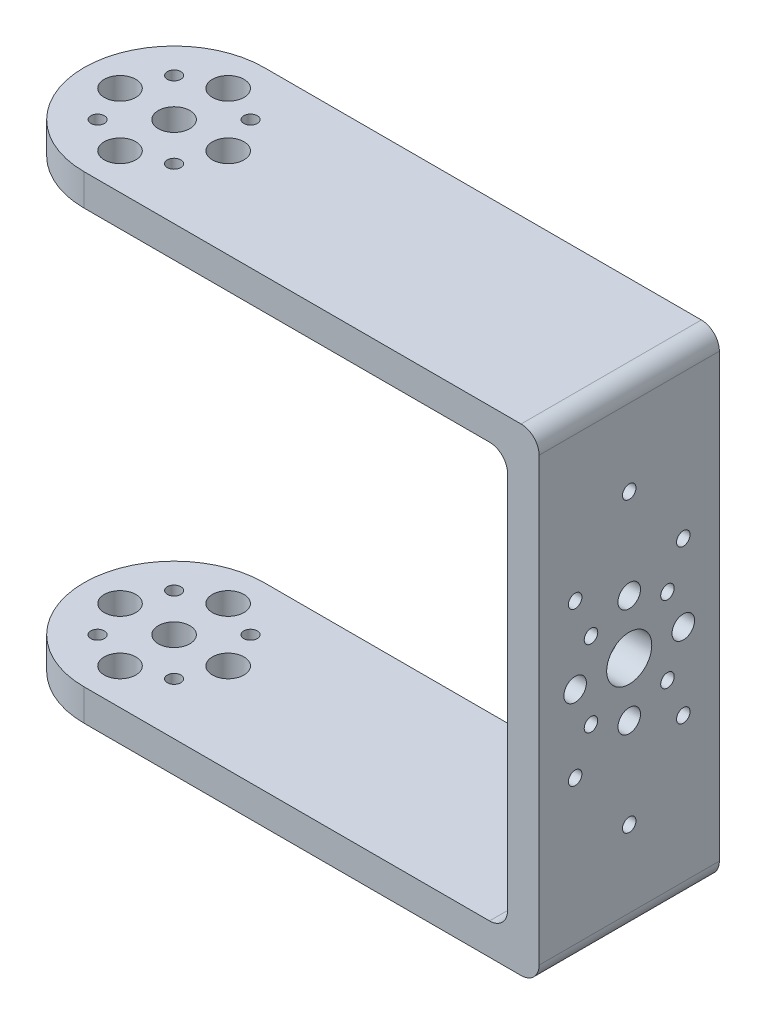
SolidWorks part; units mm, degrees
material "45"
ref_plane "Front Plane" through (0, 0, 0) normal (0, 0, 1) x (1, 0, 0)
ref_plane "Top Plane" through (0, 0, 0) normal (0, 1, 0) x (1, 0, 0)
ref_plane "Right Plane" through (0, 0, 0) normal (1, 0, 0) x (0, 0, -1)
sketch "Sketch2" plane through (0, 0, 0) normal (0, 0, 1) x (1, 0, 0)
  line L0 (4.8689, 24.8459) -> (4.8689, 28.3459)
  line L2 (4.8689, 28.3459) -> (65.3689, 28.3459)
  line L3 (4.8689, 24.8459) -> (61.8689, 24.8459)
  line L4 (4.8689, -21.1541) -> (4.8689, -24.6541)
  line L6 (4.8689, -21.1541) -> (61.8689, -21.1541)
  line L7 (4.8689, -24.6541) -> (65.3689, -24.6541)
  line L8 (65.3689, -24.6541) -> (65.3689, 28.3459)
  line L9 (61.8689, 24.8459) -> (61.8689, -21.1541)
  dimension "D1" = 3.5
  dimension "D2" = 3.5
  dimension "D3" = 3.5
  dimension "D4" = 57
extrude "Boss-Extrude1" add sketch "Sketch2" against normal blind 20
sketch "Sketch3" plane through (0, 28.3459, 0) normal (0, 1, 0) x (1, 0, 0)
  line L0 (4.8689, 10) -> (25.951, 10) construction
  line L1 (4.8689, 20) -> (4.8689, 0) construction
  line L2 (14.8689, 20) -> (4.8689, 20)
  line L3 (4.8689, 20) -> (4.8689, 10)
  line L4 (4.8689, 10) -> (4.8689, 0)
  line L5 (4.8689, 0) -> (14.8689, 0)
  arc A0 (14.8689, 20) -> (14.8689, 0) centre (14.8689, 10) ccw
  line M2 (4.8689, 0) -> (65.3689, 0)
  line M4 (65.3689, 20) -> (4.8689, 20)
  line M5 (4.8689, 20) -> (4.8689, 0)
extrude "Cut-Extrude1" cut sketch "Sketch3" against normal through all contours A0 M5 M2 | A0 M4 M5
sketch "Sketch5" plane through (0, 28.3459, 0) normal (0, 1, 0) x (1, 0, 0)
  circle A0 centre (14.8689, 10) radius 1.75
  circle A1 centre (14.8689, 10) radius 6 construction
  circle A2 centre (20.8689, 10) radius 1.75
  circle A3 centre (14.8689, 4) radius 1.75
  circle A4 centre (8.8689, 10) radius 1.75
  circle A5 centre (14.8689, 16) radius 1.75
  circle A6 centre (19.1115, 5.7574) radius 0.75
  circle A7 centre (10.6262, 5.7574) radius 0.75
  circle A8 centre (10.6262, 14.2426) radius 0.75
  circle A9 centre (19.1115, 14.2426) radius 0.75
  point P15 (14.8689, 10)
  point P24 (14.8689, 10)
  dimension "D1" = 3.5
  dimension "D2" = 12
  dimension "D3" = 3.5
  dimension "D5" = 1.5
  dimension "D4" = 4
  dimension "D6" = 4
extrude "Cut-Extrude2" cut sketch "Sketch5" against normal through all
fillet "Fillet1" radius 2 2 edges at (65.3689, -24.6541, -10) (65.3689, 28.3459, -10)
sketch "Sketch6" plane through (65.3689, 0, 0) normal (1, 0, 0) x (0, 0, -1)
  line L0 (0, 1.8459) -> (20, 1.8459) construction
  line L1 (0, -22.6541) -> (0, 26.3459) construction
  line L2 (20, -22.6541) -> (20, 26.3459) construction
  circle A0 centre (10, 1.8459) radius 6 construction
  circle A1 centre (10, 1.8459) radius 2.5
  circle A2 centre (10, 7.8459) radius 1.25
  circle A3 centre (16, 1.8459) radius 1.25
  circle A4 centre (10, -4.1541) radius 1.25
  circle A5 centre (4, 1.8459) radius 1.25
  circle A6 centre (14.2426, 6.0885) radius 0.75
  circle A7 centre (14.2426, -2.3968) radius 0.75
  circle A8 centre (5.7574, -2.3968) radius 0.75
  circle A9 centre (5.7574, 6.0885) radius 0.75
  point P20 (10, 1.8459)
  point P29 (10, 1.8459)
  dimension "D1" = 12
  dimension "D2" = 5
  dimension "D3" = 2.5
  dimension "D5" = 1.5
  dimension "D4" = 4
  dimension "D6" = 4
extrude "Cut-Extrude3" cut sketch "Sketch6" against normal blind 20
sketch "Sketch7" plane through (65.3689, 0, 0) normal (1, 0, 0) x (0, 0, -1)
  line L1 (16, -6.6541) -> (4, -6.6541) construction
  line L2 (16, -6.6541) -> (16, 10.3459) construction
  line L3 (16, 10.3459) -> (4, 10.3459) construction
  line L4 (4, -6.6541) -> (4, 10.3459) construction
  line L5 (16, -6.6541) -> (4, 10.3459) construction
  line L6 (16, 10.3459) -> (4, -6.6541) construction
  circle A0 centre (16, 10.3459) radius 0.75
  circle A1 centre (4, 10.3459) radius 0.75
  circle A2 centre (4, -6.6541) radius 0.75
  circle A3 centre (16, -6.6541) radius 0.75
  point P0 (10, 1.8459)
  dimension "D3" = 1.5
  dimension "D4" = 1.5
  dimension "D5" = 1.5
  dimension "D6" = 1.5
  dimension "D1" = 17
  dimension "D2" = 12
extrude "Cut-Extrude4" cut sketch "Sketch7" against normal blind 20
sketch "Sketch8" plane through (65.3689, 0, 0) normal (1, 0, 0) x (0, 0, -1)
  line L0 (10, 1.8459) -> (10, 17.8459) construction
  line L1 (10, 1.8459) -> (10, -14.1541) construction
  circle A0 centre (10, 17.8459) radius 0.75
  circle A1 centre (10, -14.1541) radius 0.75
  dimension "D3" = 1.5
  dimension "D4" = 1.5
  dimension "D1" = 16
  dimension "D2" = 16
extrude "Cut-Extrude5" cut sketch "Sketch8" against normal blind 20
fillet "Fillet2" radius 2 2 edges at (61.8689, 24.8459, -10) (61.8689, -21.1541, -10)
